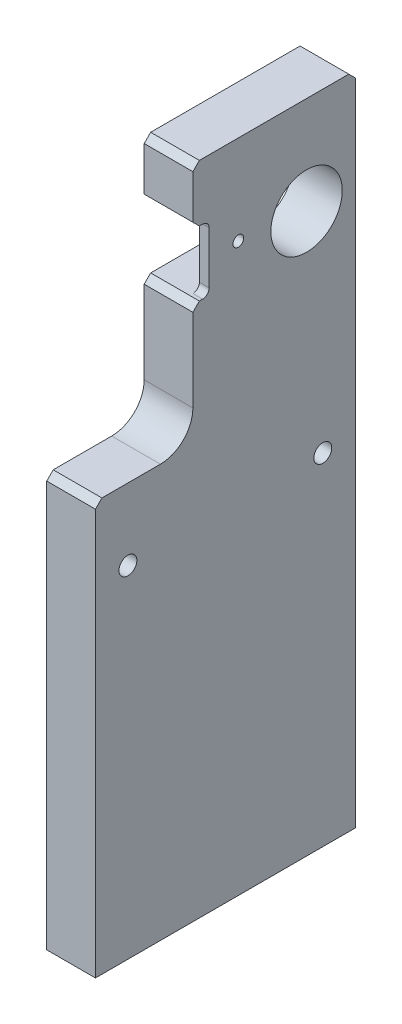
from build123d import *

# Parameters (mm, degrees)
EXTRUDE_1_DEPTH                = 7.5
SKETCH_2_R                     = 11
CUT_EXTRUDE_1_DEPTH            = 110.66312051
HOLE_WIZARD_M5_1_D             = 4.2
HOLE_WIZARD_M5_1_DEPTH         = 12.4
HOLE_WIZARD_M5_1_TIP           = 1.2618073
HOLE_WIZARD_M5_1_2_D           = 5.5
HOLE_WIZARD_M5_1_2_CBORE_D     = 10
HOLE_WIZARD_M5_1_2_CBORE_DEPTH = 5.7
HOLE_WIZARD_M6_1_D             = 5
HOLE_WIZARD_M6_1_DEPTH         = 15
HOLE_WIZARD_M6_1_TIP           = 1.502151548
CHAMFER_1_SIZE                 = 2
SKETCH_12_R                    = 2.5
CUT_EXTRUDE_2_DEPTH            = 110.66312051
HOLE_WIZARD_M4_1_D             = 3.3
SKETCH_15_W                    = 22
SKETCH_15_H                    = 20
CUT_EXTRUDE_3_DEPTH            = 12
SKETCH_16_W                    = 5
SKETCH_16_H                    = 20
CUT_EXTRUDE_4_DEPTH            = 110.293183685
SKETCH_17_R                    = 1
CUT_EXTRUDE_5_DEPTH            = 12
CHAMFER_2_SIZE                 = 2
FILLET_2_R                     = 2


with BuildPart() as part:
    # 草图1 → 凸台-拉伸1 (new, symmetric)
    with BuildSketch(Plane(origin=(0, 0, 0), x_dir=(0, 0, -1), z_dir=(1, 0, 0))):
        with BuildLine():
            Line((-10, 101), (-10, 36))
            ThreePointArc((-10, 36), (-12.928932188, 28.928932188), (-20, 26))
            Line((-20, 26), (-40, 26))
            Line((-40, 26), (-40, -101))
            Line((-40, -101), (40, -101))
            Line((40, -101), (40, 101))
            Line((40, 101), (-10, 101))
        make_face()
    extrude(amount=EXTRUDE_1_DEPTH, both=True)

    # 草图2 → 切除-拉伸1 (cut, through all)
    with BuildSketch(Plane.ZY.offset(7.5)):
        with Locations((-25, 71)):
            Circle(SKETCH_2_R)
    extrude(amount=-CUT_EXTRUDE_1_DEPTH, mode=Mode.SUBTRACT)

    # Hole Wizard M5 _1
    with Locations(Plane(origin=(0, -101, 0), x_dir=(-1, 0, 0), z_dir=(0, -1, 0))):
        with Locations((0, 25), (0, -25)):
            Hole(HOLE_WIZARD_M5_1_D / 2, depth=HOLE_WIZARD_M5_1_DEPTH)
            with Locations((0, 0, -(HOLE_WIZARD_M5_1_DEPTH + HOLE_WIZARD_M5_1_TIP / 2))):  # 118° drill point
                Cone(0, HOLE_WIZARD_M5_1_D / 2, HOLE_WIZARD_M5_1_TIP, mode=Mode.SUBTRACT)

    # Hole Wizard M5 _1 2 (through all)
    with Locations(Plane.ZY.offset(7.5)):
        with Locations((-30, 4), (30, 4)):
            CounterBoreHole(HOLE_WIZARD_M5_1_2_D / 2, HOLE_WIZARD_M5_1_2_CBORE_D / 2, HOLE_WIZARD_M5_1_2_CBORE_DEPTH)

    # M6 螺纹孔1
    with Locations(Plane(origin=(0, 0, -40), x_dir=(-1, 0, 0), z_dir=(0, 0, -1))):
        with Locations((0, 51), (0, 91)):
            Hole(HOLE_WIZARD_M6_1_D / 2, depth=HOLE_WIZARD_M6_1_DEPTH)
            with Locations((0, 0, -(HOLE_WIZARD_M6_1_DEPTH + HOLE_WIZARD_M6_1_TIP / 2))):  # 118° drill point
                Cone(0, HOLE_WIZARD_M6_1_D / 2, HOLE_WIZARD_M6_1_TIP, mode=Mode.SUBTRACT)

    # 倒角1
    chamfer_1_edges = [part.edges().sort_by_distance(p)[0] for p in [
        (0, 26, 40),
        (0, 101, 10),
        (0, 101, -40),
    ]]
    chamfer(chamfer_1_edges, length=CHAMFER_1_SIZE)

    # 草图12 → 切除-拉伸2 (cut, through all)
    with BuildSketch(Plane(origin=(7.5, 0, 0), x_dir=(0, 0, -1), z_dir=(1, 0, 0))):
        with Locations((-11, 73.5)):
            Circle(SKETCH_12_R)
    extrude(amount=-CUT_EXTRUDE_2_DEPTH, mode=Mode.SUBTRACT)

    # M4 螺纹孔1 (through all)
    with Locations(Plane.ZY.offset(7.5)):
        with Locations((-4, 73.5)):
            Hole(HOLE_WIZARD_M4_1_D / 2)

    # 草图15 → 切除-拉伸3 (cut)
    with BuildSketch(Plane.ZY.offset(7.5)):
        with Locations((-1, 73.5)):
            Rectangle(SKETCH_15_W, SKETCH_15_H)
    extrude(amount=-CUT_EXTRUDE_3_DEPTH, mode=Mode.SUBTRACT)

    # 草图16 → 切除-拉伸4 (cut, through all)
    with BuildSketch(Plane.ZY.offset(-4.5)):
        with Locations((7.5, 73.5)):
            Rectangle(SKETCH_16_W, SKETCH_16_H)
    extrude(amount=-CUT_EXTRUDE_4_DEPTH, mode=Mode.SUBTRACT)

    # 草图17 → 切除-拉伸5 (cut)
    with BuildSketch(Plane.ZY.offset(7.5)):
        with Locations((-12, 83.5)):
            Circle(SKETCH_17_R)
        with Locations((-12, 63.5)):
            Circle(SKETCH_17_R)
    extrude(amount=-CUT_EXTRUDE_5_DEPTH, mode=Mode.SUBTRACT)

    # 倒角2
    chamfer_2_edges = [part.edges().sort_by_distance(p)[0] for p in [
        (0, 83.5, 10),
        (0, 63.5, 10),
    ]]
    chamfer(chamfer_2_edges, length=CHAMFER_2_SIZE)

    # 圆角2
    fillet_2_edges = [part.edges().sort_by_distance(p)[0] for p in [
        (6, 63.5, 5),
        (6, 83.5, 5),
    ]]
    fillet(fillet_2_edges, radius=FILLET_2_R)


solid = part.part
